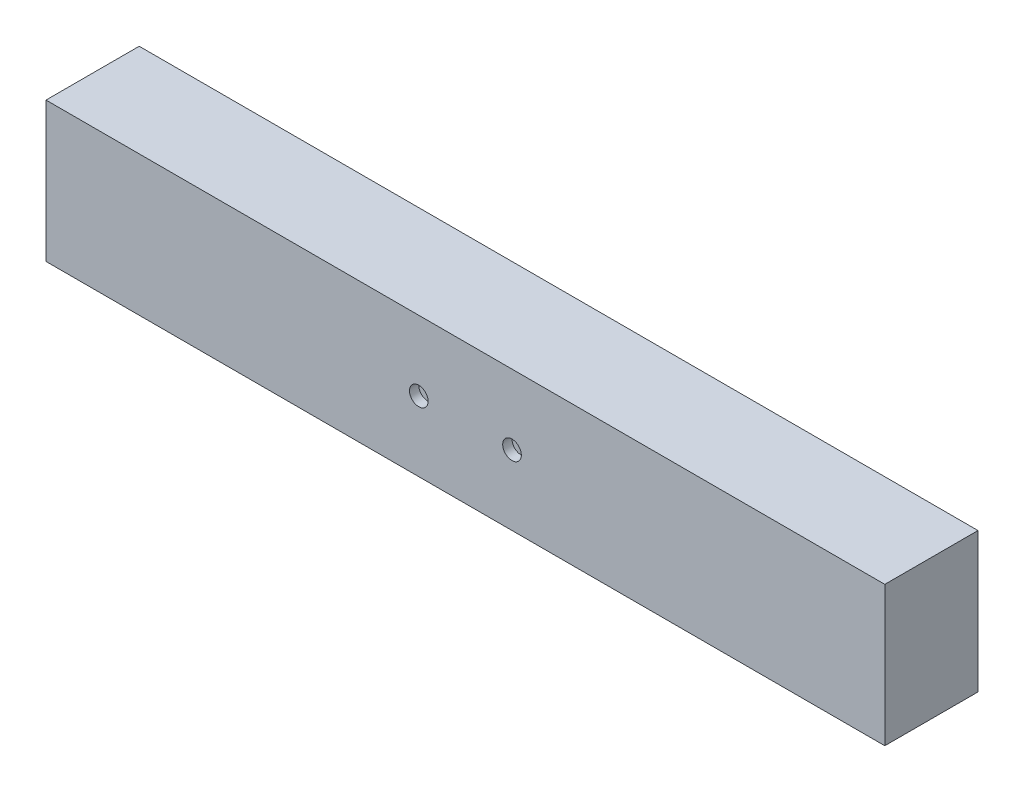
SolidWorks part; units mm, degrees
ref_plane "前视基准面" through (0, 0, 0) normal (0, 0, 1) x (1, 0, 0)
ref_plane "上视基准面" through (0, 0, 0) normal (0, 1, 0) x (1, 0, 0)
ref_plane "右视基准面" through (0, 0, 0) normal (1, 0, 0) x (0, 0, -1)
sketch "草图1" plane through (0, 0, 0) normal (0, 0, 1) x (1, 0, 0)
  line L1 (90, -15) -> (-90, -15)
  line L2 (90, -15) -> (90, 15)
  line L3 (90, 15) -> (-90, 15)
  line L4 (-90, -15) -> (-90, 15)
  line L5 (90, -15) -> (-90, 15) construction
  line L6 (90, 15) -> (-90, -15) construction
  point P0 (0, 0)
  dimension "D1" = 180
  dimension "D2" = 30
extrude "凸台-拉伸1" add sketch "草图1" along normal blind 20
sketch "草图2" plane through (0, 0, 20) normal (0, 0, 1) x (1, 0, 0)
  line L0 (-10, 0) -> (0, 0) construction
  line L1 (0, 0) -> (10, 0) construction
  circle A0 centre (-10, 0) radius 2
  circle A1 centre (10, 0) radius 2
  dimension "D2" = 4
  dimension "D1" = 10
extrude "切除-拉伸1" cut sketch "草图2" against normal blind 2
